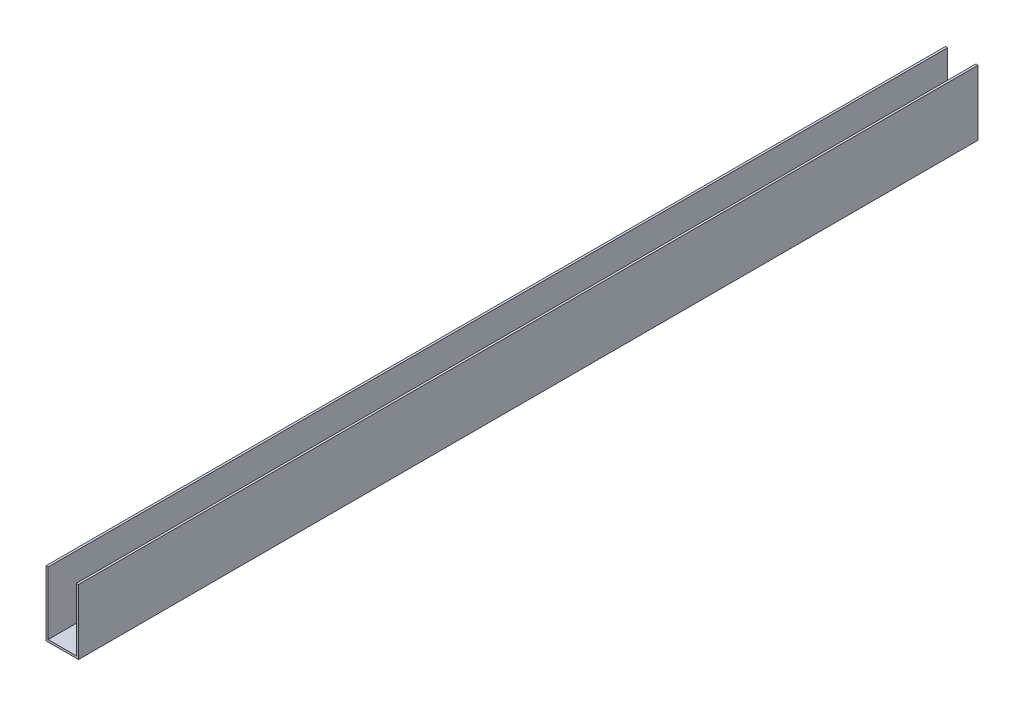
SolidWorks part; units mm, degrees
material "标准件"
ref_plane "前视基准面" through (0, 0, 0) normal (0, 0, 1) x (1, 0, 0)
ref_plane "上视基准面" through (0, 0, 0) normal (0, 1, 0) x (1, 0, 0)
ref_plane "右视基准面" through (0, 0, 0) normal (1, 0, 0) x (0, 0, -1)
sketch "草图1" plane through (0, 0, 0) normal (0, 0, 1) x (1, 0, 0)
  line L0 (0, 0) -> (0, 33.955) construction
  line L2 (-15, -30) -> (15, -30)
  line L3 (-15, -30) -> (-15, 30)
  line L4 (-15, 30) -> (15, 30)
  line L5 (15, -30) -> (15, 30)
  line L6 (-15, -30) -> (15, 30) construction
  line L7 (-15, 30) -> (15, -30) construction
  dimension "D1" = 30
  dimension "D2" = 60
extrude "凸台-拉伸1" add sketch "草图1" along normal mid plane 830
shell "抽壳1" thickness 2
